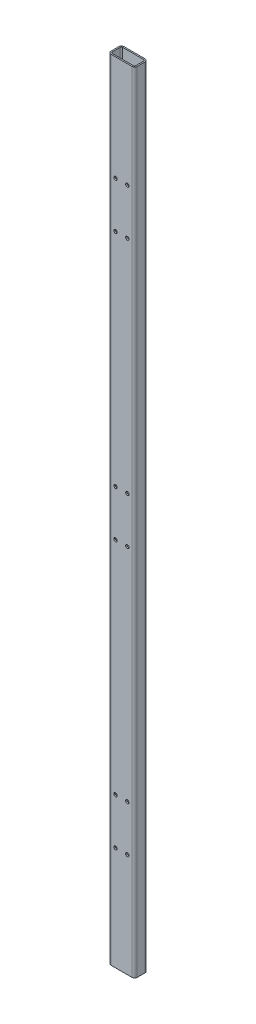
SolidWorks part; units mm, degrees
ref_plane "前视基准面" through (0, 0, 0) normal (0, 0, 1) x (1, 0, 0)
ref_plane "上视基准面" through (0, 0, 0) normal (0, 1, 0) x (1, 0, 0)
ref_plane "右视基准面" through (0, 0, 0) normal (1, 0, 0) x (0, 0, -1)
sketch "草图1" plane through (0, 0, 0) normal (1, 0, 0) x (0, 0, -1)
  line L0 (0, 0) -> (0, 1200)
  dimension "D1" = 1200
other "矩型管 40X20X2(1)"
ref_plane "基准面1" through (0, 0, 0) normal (0, 1, 0) x (0, 0, 1)
sketch "Sketch1" plane through (0, 0, 0) normal (0, 1, 0) x (0, 0, 1)
  line L0 (-6, -18) -> (6, -18)
  line L1 (-8, -16) -> (-8, 16)
  line L2 (6, 18) -> (-6, 18)
  line L3 (8, 16) -> (8, -16)
  line L4 (-6, -20) -> (6, -20)
  line L5 (-10, -16) -> (-10, 16)
  line L6 (6, 20) -> (-6, 20)
  line L7 (10, 16) -> (10, -16)
  arc A0 (10, 16) -> (6, 20) centre (6, 16) ccw
  arc A1 (6, -20) -> (10, -16) centre (6, -16) ccw
  arc A2 (-10, -16) -> (-6, -20) centre (-6, -16) ccw
  arc A3 (-6, 20) -> (-10, 16) centre (-6, 16) ccw
  arc A4 (-6, 18) -> (-8, 16) centre (-6, 16) ccw
  arc A5 (8, 16) -> (6, 18) centre (6, 16) ccw
  arc A6 (6, -18) -> (8, -16) centre (6, -16) ccw
  arc A7 (-8, -16) -> (-6, -18) centre (-6, -16) ccw
  point P0 (0, 20)
  point P1 (10, 0)
  point P2 (0, -20)
  point P3 (-10, 0)
  point P4 (-10, 20)
  point P5 (10, 20)
  point P6 (10, -20)
  point P7 (-10, -20)
  point P8 (0, 0)
  point P33 (0, 0)
hole_wizard "Ø5.2 (5.2) 直径孔1" positions "草图2" profile "草图3" hole size "Ø5.2" standard "GB" end condition through all
sketch "草图2" plane through (0, 0, -10) normal (0, 0, -1) x (-1, 0, 0)
  line L0 (0, 1200) -> (0, 1377.0022) construction
  line L1 (-16, 1200) -> (16, 1200) construction
  line L2 (0, 0) -> (0, 1200) construction
  point P0 (-9, 1040)
  point P2 (9, 1040)
  point P13 (9, 970)
  point P15 (-9, 970)
  dimension "D1" = 160
  dimension "D2" = 18
  dimension "D3" = 70
sketch "草图3" plane through (9, 1040, -10) normal (1, 0, 0) x (0, 1, 0)
  line L0 (0, 0) -> (0, 20)
  line L1 (0, 20) -> (2.6, 20)
  line L2 (2.6, 20) -> (2.6, 0)
  line L5 (2.6, 0) -> (0, 0)
  line L11 (0, -6.35) -> (0, 107.95) construction
  dimension "通孔孔直径" = 5.2
  dimension "通孔孔深度" = 20
pattern_linear "阵列(线性)1" count 3 spacing 406 along (0, -1, 0) of "Ø5.2 (5.2) 直径孔1"
equation "\"D1@Sketch1\" = \"Thickness@Sketch1\" * 2"
